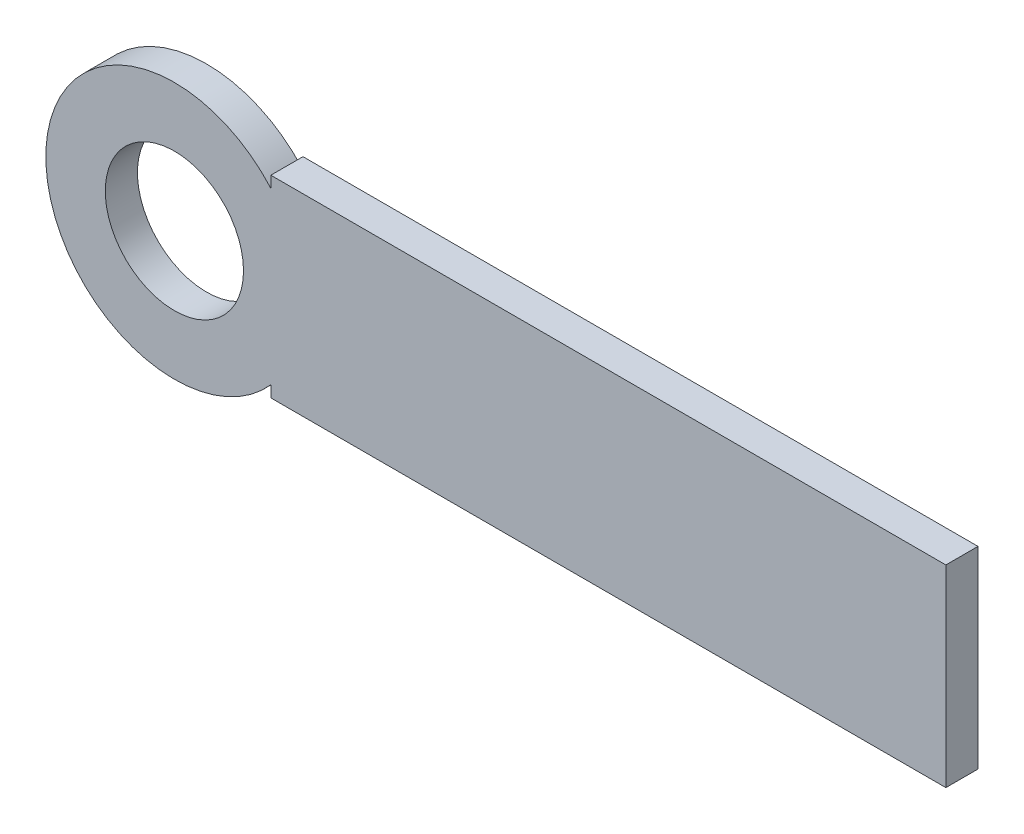
SolidWorks part; units mm, degrees
ref_plane "前视基准面" through (0, 0, 0) normal (0, 0, 1) x (1, 0, 0)
ref_plane "上视基准面" through (0, 0, 0) normal (0, 1, 0) x (1, 0, 0)
ref_plane "右视基准面" through (0, 0, 0) normal (1, 0, 0) x (0, 0, -1)
other "Configuration Table"
sketch "草图1" plane through (0, 0, 0) normal (0, 0, 1) x (1, 0, 0)
  circle A0 centre (0, 0) radius 4
  circle A1 centre (0, 0) radius 2.15
  point P0 (0, 0)
  dimension "D1" = 4.3
  dimension "D2" = 8
extrude "凸台-拉伸1" add sketch "草图1" against normal mid plane 1
sketch "草图2" plane through (0, 0, 0) normal (0, 0, 1) x (1, 0, 0)
  line L0 (3, -3) -> (24, -3)
  line L1 (24, -3) -> (24, 3)
  line L2 (24, 3) -> (3, 3)
  line L3 (3, 3) -> (3, -3)
  point P0 (0, 0)
  dimension "D1" = 21
  dimension "D2" = 24
  dimension "D3" = 3
  dimension "D4" = 6
extrude "凸台-拉伸2" add sketch "草图2" against normal mid plane 1
